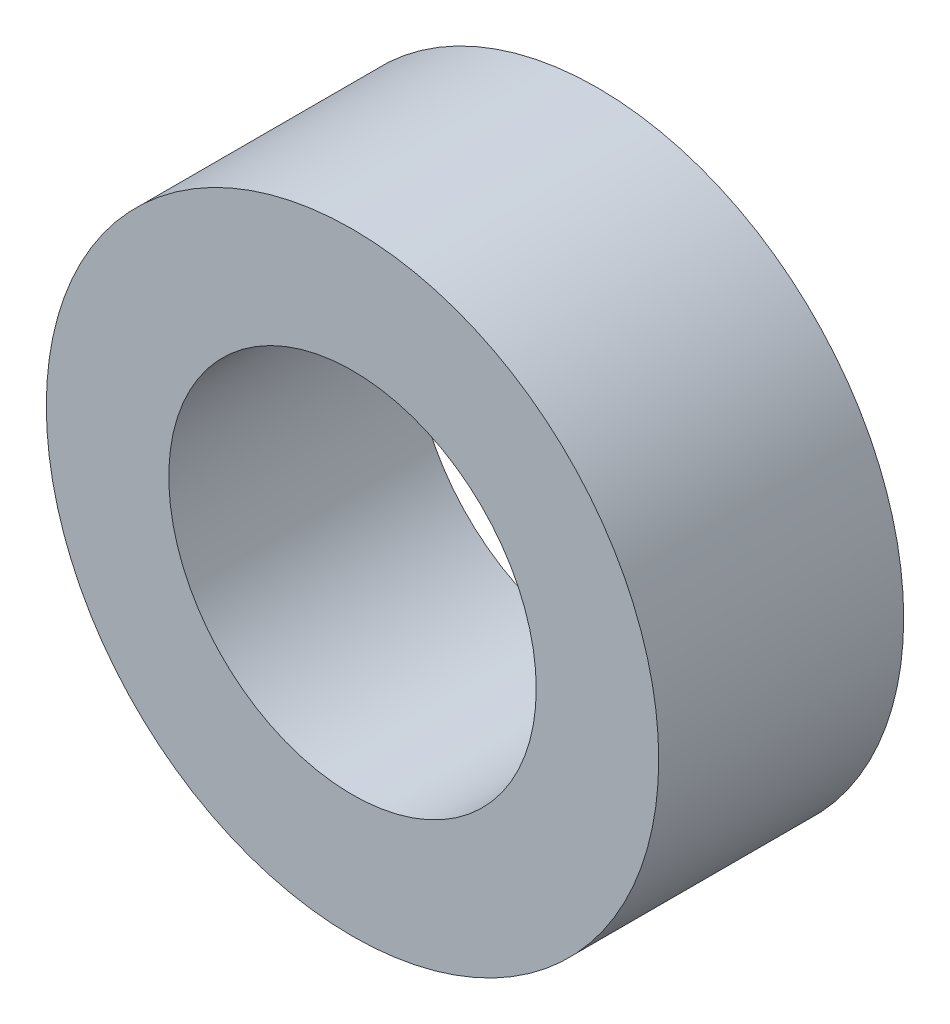
from build123d import *

# Parameters (mm, degrees)
SKETCH1_R           = 5
SKETCH1_R_2         = 3
BOSS_EXTRUDE1_DEPTH = 4


with BuildPart() as part:
    # Sketch1 → Boss-Extrude1 (new body)
    with BuildSketch(Plane.XY):
        Circle(SKETCH1_R)
        Circle(SKETCH1_R_2, mode=Mode.SUBTRACT)
    extrude(amount=BOSS_EXTRUDE1_DEPTH)


solid = part.part
